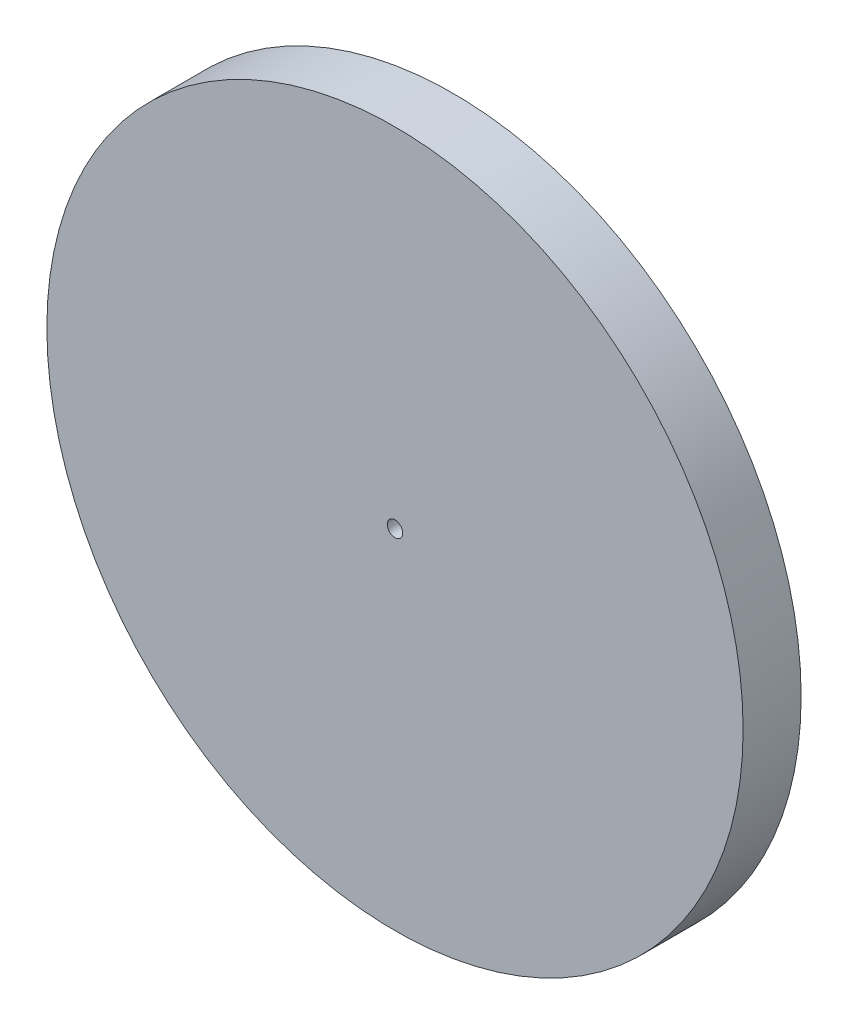
from build123d import *

# Parameters (mm, degrees)
SKETCH1_R           = 900
BOSS_EXTRUDE1_DEPTH = 150
SKETCH2_R           = 20
CUT_EXTRUDE1_DEPTH  = 1282.600561798


with BuildPart() as part:
    # Sketch1 → Boss-Extrude1 (new body)
    with BuildSketch(Plane.XY):
        Circle(SKETCH1_R)
    extrude(amount=BOSS_EXTRUDE1_DEPTH)

    # Sketch2 → Cut-Extrude1 (cut, through all)
    with BuildSketch(Plane(origin=(0, 0, 0), x_dir=(-1, 0, 0), z_dir=(0, 0, -1))):
        Circle(SKETCH2_R)
    extrude(amount=-CUT_EXTRUDE1_DEPTH, mode=Mode.SUBTRACT)


solid = part.part
